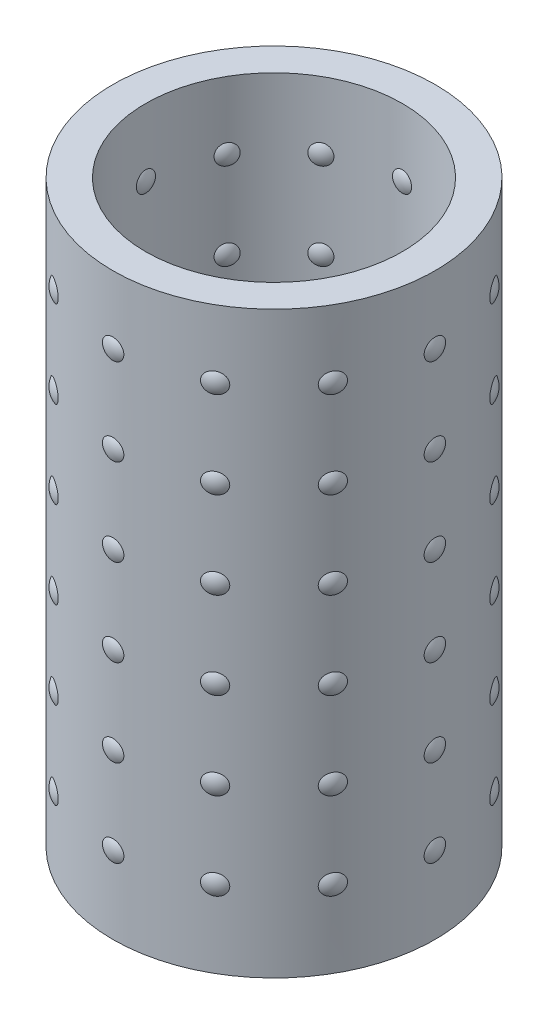
from build123d import *

# Parameters (mm, degrees)
SKETCH1_R           = 8.35
SKETCH1_R_2         = 6.65
BOSS_EXTRUDE1_DEPTH = 30
LPATTERN5_COUNT     = 8
LPATTERN5_PITCH     = 4.5
CIRPATTERN1_COUNT   = 12


with BuildPart() as part:
    # Sketch1 → Boss-Extrude1 (new body)
    with BuildSketch(Plane(origin=(0, 0, 0), x_dir=(1, 0, 0), z_dir=(0, 1, 0))):
        with Locations(Location((0, 0, 0), (0, 0, 270))):
            Circle(SKETCH1_R)
        with Locations(Location((0, 0, 0), (0, 0, 270))):
            Circle(SKETCH1_R_2, mode=Mode.SUBTRACT)
    extrude(amount=BOSS_EXTRUDE1_DEPTH)

    # Sketch2 → Revolve3 (revolve)
    with BuildSketch(Plane(origin=(0, 0, 0), x_dir=(0, 0, -1), z_dir=(1, 0, 0))):
        with BuildLine():
            Line((-8.5, 4), (-6.5, 4))
            ThreePointArc((-6.5, 4), (-7.5, 5), (-8.5, 4))
        make_face()
    revolve3 = revolve(axis=Axis((0, 4, 8.5), (0, 0, -1)))

    # LPattern5: Revolve3 ×8, 2 skipped
    with Locations(*[(0, i * LPATTERN5_PITCH, 0) for i in range(1, LPATTERN5_COUNT) if i not in (6, 7)]):
        add(revolve3)

    # CirPattern1: Revolve3 ×12 about axis
    cirpattern1_axis = Axis((0, 0, 0), (0, 1, 0))
    for i in range(1, CIRPATTERN1_COUNT):
        add(revolve3.rotate(cirpattern1_axis, i * 360 / CIRPATTERN1_COUNT))

    # CirPattern1 copy 1 sketch → CirPattern1 copy 1 (revolve)
    with BuildSketch(Plane(origin=(0, 4.5, 0), x_dir=(-0.49999999999999994, 0, -0.8660254037844387), z_dir=(0.8660254037844387, 0, -0.49999999999999994))):
        with BuildLine():
            Line((-8.5, 4), (-6.5, 4))
            ThreePointArc((-6.5, 4), (-7.5, 5), (-8.5, 4))
        make_face()
    revolve(axis=Axis((4.25, 8.5, 7.361215932), (-0.49999999999999994, 0, -0.8660254037844387)))

    # CirPattern1 copy 2 sketch → CirPattern1 copy 2 (revolve)
    with BuildSketch(Plane(origin=(0, 4.5, 0), x_dir=(-0.8660254037844386, 0, -0.5000000000000001), z_dir=(0.5000000000000001, 0, -0.8660254037844386))):
        with BuildLine():
            Line((-8.5, 4), (-6.5, 4))
            ThreePointArc((-6.5, 4), (-7.5, 5), (-8.5, 4))
        make_face()
    revolve(axis=Axis((7.361215932, 8.5, 4.25), (-0.8660254037844386, 0, -0.5000000000000001)))

    # CirPattern1 copy 3 sketch → CirPattern1 copy 3 (revolve)
    with BuildSketch(Plane(origin=(0, 4.5, 0), x_dir=(-1, 0, 0), z_dir=(0, 0, -1))):
        with BuildLine():
            Line((-8.5, 4), (-6.5, 4))
            ThreePointArc((-6.5, 4), (-7.5, 5), (-8.5, 4))
        make_face()
    revolve(axis=Axis((8.5, 8.5, 0), (-1, 0, 0)))

    # CirPattern1 copy 4 sketch → CirPattern1 copy 4 (revolve)
    with BuildSketch(Plane(origin=(0, 4.5, 0), x_dir=(-0.8660254037844387, 0, 0.4999999999999998), z_dir=(-0.4999999999999998, 0, -0.8660254037844387))):
        with BuildLine():
            Line((-8.5, 4), (-6.5, 4))
            ThreePointArc((-6.5, 4), (-7.5, 5), (-8.5, 4))
        make_face()
    revolve(axis=Axis((7.361215932, 8.5, -4.25), (-0.8660254037844387, 0, 0.4999999999999998)))

    # CirPattern1 copy 5 sketch → CirPattern1 copy 5 (revolve)
    with BuildSketch(Plane(origin=(0, 4.5, 0), x_dir=(-0.49999999999999994, 0, 0.8660254037844387), z_dir=(-0.8660254037844387, 0, -0.49999999999999994))):
        with BuildLine():
            Line((-8.5, 4), (-6.5, 4))
            ThreePointArc((-6.5, 4), (-7.5, 5), (-8.5, 4))
        make_face()
    revolve(axis=Axis((4.25, 8.5, -7.361215932), (-0.49999999999999994, 0, 0.8660254037844387)))

    # CirPattern1 copy 6 sketch → CirPattern1 copy 6 (revolve)
    with BuildSketch(Plane(origin=(0, 4.5, 0), x_dir=(0, 0, 1), z_dir=(-1, 0, 0))):
        with BuildLine():
            Line((-8.5, 4), (-6.5, 4))
            ThreePointArc((-6.5, 4), (-7.5, 5), (-8.5, 4))
        make_face()
    revolve(axis=Axis((0, 8.5, -8.5), (0, 0, 1)))

    # CirPattern1 copy 7 sketch → CirPattern1 copy 7 (revolve)
    with BuildSketch(Plane(origin=(0, 4.5, 0), x_dir=(0.5000000000000001, 0, 0.8660254037844386), z_dir=(-0.8660254037844386, 0, 0.5000000000000001))):
        with BuildLine():
            Line((-8.5, 4), (-6.5, 4))
            ThreePointArc((-6.5, 4), (-7.5, 5), (-8.5, 4))
        make_face()
    revolve(axis=Axis((-4.25, 8.5, -7.361215932), (0.5000000000000001, 0, 0.8660254037844386)))

    # CirPattern1 copy 8 sketch → CirPattern1 copy 8 (revolve)
    with BuildSketch(Plane(origin=(0, 4.5, 0), x_dir=(0.8660254037844384, 0, 0.5000000000000004), z_dir=(-0.5000000000000004, 0, 0.8660254037844384))):
        with BuildLine():
            Line((-8.5, 4), (-6.5, 4))
            ThreePointArc((-6.5, 4), (-7.5, 5), (-8.5, 4))
        make_face()
    revolve(axis=Axis((-7.361215932, 8.5, -4.25), (0.8660254037844384, 0, 0.5000000000000004)))

    # CirPattern1 copy 9 sketch → CirPattern1 copy 9 (revolve)
    with BuildSketch(Plane(origin=(0, 4.5, 0), x_dir=(1, 0, 0), z_dir=(0, 0, 1))):
        with BuildLine():
            Line((-8.5, 4), (-6.5, 4))
            ThreePointArc((-6.5, 4), (-7.5, 5), (-8.5, 4))
        make_face()
    revolve(axis=Axis((-8.5, 8.5, 0), (1, 0, 0)))

    # CirPattern1 copy 10 sketch → CirPattern1 copy 10 (revolve)
    with BuildSketch(Plane(origin=(0, 4.5, 0), x_dir=(0.8660254037844386, 0, -0.5000000000000001), z_dir=(0.5000000000000001, 0, 0.8660254037844386))):
        with BuildLine():
            Line((-8.5, 4), (-6.5, 4))
            ThreePointArc((-6.5, 4), (-7.5, 5), (-8.5, 4))
        make_face()
    revolve(axis=Axis((-7.361215932, 8.5, 4.25), (0.8660254037844386, 0, -0.5000000000000001)))

    # CirPattern1 copy 11 sketch → CirPattern1 copy 11 (revolve)
    with BuildSketch(Plane(origin=(0, 4.5, 0), x_dir=(0.5000000000000004, 0, -0.8660254037844384), z_dir=(0.8660254037844384, 0, 0.5000000000000004))):
        with BuildLine():
            Line((-8.5, 4), (-6.5, 4))
            ThreePointArc((-6.5, 4), (-7.5, 5), (-8.5, 4))
        make_face()
    revolve(axis=Axis((-4.25, 8.5, 7.361215932), (0.5000000000000004, 0, -0.8660254037844384)))

    # CirPattern1 copy 12 sketch → CirPattern1 copy 12 (revolve)
    with BuildSketch(Plane(origin=(0, 9, 0), x_dir=(-0.49999999999999994, 0, -0.8660254037844387), z_dir=(0.8660254037844387, 0, -0.49999999999999994))):
        with BuildLine():
            Line((-8.5, 4), (-6.5, 4))
            ThreePointArc((-6.5, 4), (-7.5, 5), (-8.5, 4))
        make_face()
    revolve(axis=Axis((4.25, 13, 7.361215932), (-0.49999999999999994, 0, -0.8660254037844387)))

    # CirPattern1 copy 13 sketch → CirPattern1 copy 13 (revolve)
    with BuildSketch(Plane(origin=(0, 9, 0), x_dir=(-0.8660254037844386, 0, -0.5000000000000001), z_dir=(0.5000000000000001, 0, -0.8660254037844386))):
        with BuildLine():
            Line((-8.5, 4), (-6.5, 4))
            ThreePointArc((-6.5, 4), (-7.5, 5), (-8.5, 4))
        make_face()
    revolve(axis=Axis((7.361215932, 13, 4.25), (-0.8660254037844386, 0, -0.5000000000000001)))

    # CirPattern1 copy 14 sketch → CirPattern1 copy 14 (revolve)
    with BuildSketch(Plane(origin=(0, 9, 0), x_dir=(-1, 0, 0), z_dir=(0, 0, -1))):
        with BuildLine():
            Line((-8.5, 4), (-6.5, 4))
            ThreePointArc((-6.5, 4), (-7.5, 5), (-8.5, 4))
        make_face()
    revolve(axis=Axis((8.5, 13, 0), (-1, 0, 0)))

    # CirPattern1 copy 15 sketch → CirPattern1 copy 15 (revolve)
    with BuildSketch(Plane(origin=(0, 9, 0), x_dir=(-0.8660254037844387, 0, 0.4999999999999998), z_dir=(-0.4999999999999998, 0, -0.8660254037844387))):
        with BuildLine():
            Line((-8.5, 4), (-6.5, 4))
            ThreePointArc((-6.5, 4), (-7.5, 5), (-8.5, 4))
        make_face()
    revolve(axis=Axis((7.361215932, 13, -4.25), (-0.8660254037844387, 0, 0.4999999999999998)))

    # CirPattern1 copy 16 sketch → CirPattern1 copy 16 (revolve)
    with BuildSketch(Plane(origin=(0, 9, 0), x_dir=(-0.49999999999999994, 0, 0.8660254037844387), z_dir=(-0.8660254037844387, 0, -0.49999999999999994))):
        with BuildLine():
            Line((-8.5, 4), (-6.5, 4))
            ThreePointArc((-6.5, 4), (-7.5, 5), (-8.5, 4))
        make_face()
    revolve(axis=Axis((4.25, 13, -7.361215932), (-0.49999999999999994, 0, 0.8660254037844387)))

    # CirPattern1 copy 17 sketch → CirPattern1 copy 17 (revolve)
    with BuildSketch(Plane(origin=(0, 9, 0), x_dir=(0, 0, 1), z_dir=(-1, 0, 0))):
        with BuildLine():
            Line((-8.5, 4), (-6.5, 4))
            ThreePointArc((-6.5, 4), (-7.5, 5), (-8.5, 4))
        make_face()
    revolve(axis=Axis((0, 13, -8.5), (0, 0, 1)))

    # CirPattern1 copy 18 sketch → CirPattern1 copy 18 (revolve)
    with BuildSketch(Plane(origin=(0, 9, 0), x_dir=(0.5000000000000001, 0, 0.8660254037844386), z_dir=(-0.8660254037844386, 0, 0.5000000000000001))):
        with BuildLine():
            Line((-8.5, 4), (-6.5, 4))
            ThreePointArc((-6.5, 4), (-7.5, 5), (-8.5, 4))
        make_face()
    revolve(axis=Axis((-4.25, 13, -7.361215932), (0.5000000000000001, 0, 0.8660254037844386)))

    # CirPattern1 copy 19 sketch → CirPattern1 copy 19 (revolve)
    with BuildSketch(Plane(origin=(0, 9, 0), x_dir=(0.8660254037844384, 0, 0.5000000000000004), z_dir=(-0.5000000000000004, 0, 0.8660254037844384))):
        with BuildLine():
            Line((-8.5, 4), (-6.5, 4))
            ThreePointArc((-6.5, 4), (-7.5, 5), (-8.5, 4))
        make_face()
    revolve(axis=Axis((-7.361215932, 13, -4.25), (0.8660254037844384, 0, 0.5000000000000004)))

    # CirPattern1 copy 20 sketch → CirPattern1 copy 20 (revolve)
    with BuildSketch(Plane(origin=(0, 9, 0), x_dir=(1, 0, 0), z_dir=(0, 0, 1))):
        with BuildLine():
            Line((-8.5, 4), (-6.5, 4))
            ThreePointArc((-6.5, 4), (-7.5, 5), (-8.5, 4))
        make_face()
    revolve(axis=Axis((-8.5, 13, 0), (1, 0, 0)))

    # CirPattern1 copy 21 sketch → CirPattern1 copy 21 (revolve)
    with BuildSketch(Plane(origin=(0, 9, 0), x_dir=(0.8660254037844386, 0, -0.5000000000000001), z_dir=(0.5000000000000001, 0, 0.8660254037844386))):
        with BuildLine():
            Line((-8.5, 4), (-6.5, 4))
            ThreePointArc((-6.5, 4), (-7.5, 5), (-8.5, 4))
        make_face()
    revolve(axis=Axis((-7.361215932, 13, 4.25), (0.8660254037844386, 0, -0.5000000000000001)))

    # CirPattern1 copy 22 sketch → CirPattern1 copy 22 (revolve)
    with BuildSketch(Plane(origin=(0, 9, 0), x_dir=(0.5000000000000004, 0, -0.8660254037844384), z_dir=(0.8660254037844384, 0, 0.5000000000000004))):
        with BuildLine():
            Line((-8.5, 4), (-6.5, 4))
            ThreePointArc((-6.5, 4), (-7.5, 5), (-8.5, 4))
        make_face()
    revolve(axis=Axis((-4.25, 13, 7.361215932), (0.5000000000000004, 0, -0.8660254037844384)))

    # CirPattern1 copy 23 sketch → CirPattern1 copy 23 (revolve)
    with BuildSketch(Plane(origin=(0, 13.5, 0), x_dir=(-0.49999999999999994, 0, -0.8660254037844387), z_dir=(0.8660254037844387, 0, -0.49999999999999994))):
        with BuildLine():
            Line((-8.5, 4), (-6.5, 4))
            ThreePointArc((-6.5, 4), (-7.5, 5), (-8.5, 4))
        make_face()
    revolve(axis=Axis((4.25, 17.5, 7.361215932), (-0.49999999999999994, 0, -0.8660254037844387)))

    # CirPattern1 copy 24 sketch → CirPattern1 copy 24 (revolve)
    with BuildSketch(Plane(origin=(0, 13.5, 0), x_dir=(-0.8660254037844386, 0, -0.5000000000000001), z_dir=(0.5000000000000001, 0, -0.8660254037844386))):
        with BuildLine():
            Line((-8.5, 4), (-6.5, 4))
            ThreePointArc((-6.5, 4), (-7.5, 5), (-8.5, 4))
        make_face()
    revolve(axis=Axis((7.361215932, 17.5, 4.25), (-0.8660254037844386, 0, -0.5000000000000001)))

    # CirPattern1 copy 25 sketch → CirPattern1 copy 25 (revolve)
    with BuildSketch(Plane(origin=(0, 13.5, 0), x_dir=(-1, 0, 0), z_dir=(0, 0, -1))):
        with BuildLine():
            Line((-8.5, 4), (-6.5, 4))
            ThreePointArc((-6.5, 4), (-7.5, 5), (-8.5, 4))
        make_face()
    revolve(axis=Axis((8.5, 17.5, 0), (-1, 0, 0)))

    # CirPattern1 copy 26 sketch → CirPattern1 copy 26 (revolve)
    with BuildSketch(Plane(origin=(0, 13.5, 0), x_dir=(-0.8660254037844387, 0, 0.4999999999999998), z_dir=(-0.4999999999999998, 0, -0.8660254037844387))):
        with BuildLine():
            Line((-8.5, 4), (-6.5, 4))
            ThreePointArc((-6.5, 4), (-7.5, 5), (-8.5, 4))
        make_face()
    revolve(axis=Axis((7.361215932, 17.5, -4.25), (-0.8660254037844387, 0, 0.4999999999999998)))

    # CirPattern1 copy 27 sketch → CirPattern1 copy 27 (revolve)
    with BuildSketch(Plane(origin=(0, 13.5, 0), x_dir=(-0.49999999999999994, 0, 0.8660254037844387), z_dir=(-0.8660254037844387, 0, -0.49999999999999994))):
        with BuildLine():
            Line((-8.5, 4), (-6.5, 4))
            ThreePointArc((-6.5, 4), (-7.5, 5), (-8.5, 4))
        make_face()
    revolve(axis=Axis((4.25, 17.5, -7.361215932), (-0.49999999999999994, 0, 0.8660254037844387)))

    # CirPattern1 copy 28 sketch → CirPattern1 copy 28 (revolve)
    with BuildSketch(Plane(origin=(0, 13.5, 0), x_dir=(0, 0, 1), z_dir=(-1, 0, 0))):
        with BuildLine():
            Line((-8.5, 4), (-6.5, 4))
            ThreePointArc((-6.5, 4), (-7.5, 5), (-8.5, 4))
        make_face()
    revolve(axis=Axis((0, 17.5, -8.5), (0, 0, 1)))

    # CirPattern1 copy 29 sketch → CirPattern1 copy 29 (revolve)
    with BuildSketch(Plane(origin=(0, 13.5, 0), x_dir=(0.5000000000000001, 0, 0.8660254037844386), z_dir=(-0.8660254037844386, 0, 0.5000000000000001))):
        with BuildLine():
            Line((-8.5, 4), (-6.5, 4))
            ThreePointArc((-6.5, 4), (-7.5, 5), (-8.5, 4))
        make_face()
    revolve(axis=Axis((-4.25, 17.5, -7.361215932), (0.5000000000000001, 0, 0.8660254037844386)))

    # CirPattern1 copy 30 sketch → CirPattern1 copy 30 (revolve)
    with BuildSketch(Plane(origin=(0, 13.5, 0), x_dir=(0.8660254037844384, 0, 0.5000000000000004), z_dir=(-0.5000000000000004, 0, 0.8660254037844384))):
        with BuildLine():
            Line((-8.5, 4), (-6.5, 4))
            ThreePointArc((-6.5, 4), (-7.5, 5), (-8.5, 4))
        make_face()
    revolve(axis=Axis((-7.361215932, 17.5, -4.25), (0.8660254037844384, 0, 0.5000000000000004)))

    # CirPattern1 copy 31 sketch → CirPattern1 copy 31 (revolve)
    with BuildSketch(Plane(origin=(0, 13.5, 0), x_dir=(1, 0, 0), z_dir=(0, 0, 1))):
        with BuildLine():
            Line((-8.5, 4), (-6.5, 4))
            ThreePointArc((-6.5, 4), (-7.5, 5), (-8.5, 4))
        make_face()
    revolve(axis=Axis((-8.5, 17.5, 0), (1, 0, 0)))

    # CirPattern1 copy 32 sketch → CirPattern1 copy 32 (revolve)
    with BuildSketch(Plane(origin=(0, 13.5, 0), x_dir=(0.8660254037844386, 0, -0.5000000000000001), z_dir=(0.5000000000000001, 0, 0.8660254037844386))):
        with BuildLine():
            Line((-8.5, 4), (-6.5, 4))
            ThreePointArc((-6.5, 4), (-7.5, 5), (-8.5, 4))
        make_face()
    revolve(axis=Axis((-7.361215932, 17.5, 4.25), (0.8660254037844386, 0, -0.5000000000000001)))

    # CirPattern1 copy 33 sketch → CirPattern1 copy 33 (revolve)
    with BuildSketch(Plane(origin=(0, 13.5, 0), x_dir=(0.5000000000000004, 0, -0.8660254037844384), z_dir=(0.8660254037844384, 0, 0.5000000000000004))):
        with BuildLine():
            Line((-8.5, 4), (-6.5, 4))
            ThreePointArc((-6.5, 4), (-7.5, 5), (-8.5, 4))
        make_face()
    revolve(axis=Axis((-4.25, 17.5, 7.361215932), (0.5000000000000004, 0, -0.8660254037844384)))

    # CirPattern1 copy 34 sketch → CirPattern1 copy 34 (revolve)
    with BuildSketch(Plane(origin=(0, 18, 0), x_dir=(-0.49999999999999994, 0, -0.8660254037844387), z_dir=(0.8660254037844387, 0, -0.49999999999999994))):
        with BuildLine():
            Line((-8.5, 4), (-6.5, 4))
            ThreePointArc((-6.5, 4), (-7.5, 5), (-8.5, 4))
        make_face()
    revolve(axis=Axis((4.25, 22, 7.361215932), (-0.49999999999999994, 0, -0.8660254037844387)))

    # CirPattern1 copy 35 sketch → CirPattern1 copy 35 (revolve)
    with BuildSketch(Plane(origin=(0, 18, 0), x_dir=(-0.8660254037844386, 0, -0.5000000000000001), z_dir=(0.5000000000000001, 0, -0.8660254037844386))):
        with BuildLine():
            Line((-8.5, 4), (-6.5, 4))
            ThreePointArc((-6.5, 4), (-7.5, 5), (-8.5, 4))
        make_face()
    revolve(axis=Axis((7.361215932, 22, 4.25), (-0.8660254037844386, 0, -0.5000000000000001)))

    # CirPattern1 copy 36 sketch → CirPattern1 copy 36 (revolve)
    with BuildSketch(Plane(origin=(0, 18, 0), x_dir=(-1, 0, 0), z_dir=(0, 0, -1))):
        with BuildLine():
            Line((-8.5, 4), (-6.5, 4))
            ThreePointArc((-6.5, 4), (-7.5, 5), (-8.5, 4))
        make_face()
    revolve(axis=Axis((8.5, 22, 0), (-1, 0, 0)))

    # CirPattern1 copy 37 sketch → CirPattern1 copy 37 (revolve)
    with BuildSketch(Plane(origin=(0, 18, 0), x_dir=(-0.8660254037844387, 0, 0.4999999999999998), z_dir=(-0.4999999999999998, 0, -0.8660254037844387))):
        with BuildLine():
            Line((-8.5, 4), (-6.5, 4))
            ThreePointArc((-6.5, 4), (-7.5, 5), (-8.5, 4))
        make_face()
    revolve(axis=Axis((7.361215932, 22, -4.25), (-0.8660254037844387, 0, 0.4999999999999998)))

    # CirPattern1 copy 38 sketch → CirPattern1 copy 38 (revolve)
    with BuildSketch(Plane(origin=(0, 18, 0), x_dir=(-0.49999999999999994, 0, 0.8660254037844387), z_dir=(-0.8660254037844387, 0, -0.49999999999999994))):
        with BuildLine():
            Line((-8.5, 4), (-6.5, 4))
            ThreePointArc((-6.5, 4), (-7.5, 5), (-8.5, 4))
        make_face()
    revolve(axis=Axis((4.25, 22, -7.361215932), (-0.49999999999999994, 0, 0.8660254037844387)))

    # CirPattern1 copy 39 sketch → CirPattern1 copy 39 (revolve)
    with BuildSketch(Plane(origin=(0, 18, 0), x_dir=(0, 0, 1), z_dir=(-1, 0, 0))):
        with BuildLine():
            Line((-8.5, 4), (-6.5, 4))
            ThreePointArc((-6.5, 4), (-7.5, 5), (-8.5, 4))
        make_face()
    revolve(axis=Axis((0, 22, -8.5), (0, 0, 1)))

    # CirPattern1 copy 40 sketch → CirPattern1 copy 40 (revolve)
    with BuildSketch(Plane(origin=(0, 18, 0), x_dir=(0.5000000000000001, 0, 0.8660254037844386), z_dir=(-0.8660254037844386, 0, 0.5000000000000001))):
        with BuildLine():
            Line((-8.5, 4), (-6.5, 4))
            ThreePointArc((-6.5, 4), (-7.5, 5), (-8.5, 4))
        make_face()
    revolve(axis=Axis((-4.25, 22, -7.361215932), (0.5000000000000001, 0, 0.8660254037844386)))

    # CirPattern1 copy 41 sketch → CirPattern1 copy 41 (revolve)
    with BuildSketch(Plane(origin=(0, 18, 0), x_dir=(0.8660254037844384, 0, 0.5000000000000004), z_dir=(-0.5000000000000004, 0, 0.8660254037844384))):
        with BuildLine():
            Line((-8.5, 4), (-6.5, 4))
            ThreePointArc((-6.5, 4), (-7.5, 5), (-8.5, 4))
        make_face()
    revolve(axis=Axis((-7.361215932, 22, -4.25), (0.8660254037844384, 0, 0.5000000000000004)))

    # CirPattern1 copy 42 sketch → CirPattern1 copy 42 (revolve)
    with BuildSketch(Plane(origin=(0, 18, 0), x_dir=(1, 0, 0), z_dir=(0, 0, 1))):
        with BuildLine():
            Line((-8.5, 4), (-6.5, 4))
            ThreePointArc((-6.5, 4), (-7.5, 5), (-8.5, 4))
        make_face()
    revolve(axis=Axis((-8.5, 22, 0), (1, 0, 0)))

    # CirPattern1 copy 43 sketch → CirPattern1 copy 43 (revolve)
    with BuildSketch(Plane(origin=(0, 18, 0), x_dir=(0.8660254037844386, 0, -0.5000000000000001), z_dir=(0.5000000000000001, 0, 0.8660254037844386))):
        with BuildLine():
            Line((-8.5, 4), (-6.5, 4))
            ThreePointArc((-6.5, 4), (-7.5, 5), (-8.5, 4))
        make_face()
    revolve(axis=Axis((-7.361215932, 22, 4.25), (0.8660254037844386, 0, -0.5000000000000001)))

    # CirPattern1 copy 44 sketch → CirPattern1 copy 44 (revolve)
    with BuildSketch(Plane(origin=(0, 18, 0), x_dir=(0.5000000000000004, 0, -0.8660254037844384), z_dir=(0.8660254037844384, 0, 0.5000000000000004))):
        with BuildLine():
            Line((-8.5, 4), (-6.5, 4))
            ThreePointArc((-6.5, 4), (-7.5, 5), (-8.5, 4))
        make_face()
    revolve(axis=Axis((-4.25, 22, 7.361215932), (0.5000000000000004, 0, -0.8660254037844384)))

    # CirPattern1 copy 45 sketch → CirPattern1 copy 45 (revolve)
    with BuildSketch(Plane(origin=(0, 22.5, 0), x_dir=(-0.49999999999999994, 0, -0.8660254037844387), z_dir=(0.8660254037844387, 0, -0.49999999999999994))):
        with BuildLine():
            Line((-8.5, 4), (-6.5, 4))
            ThreePointArc((-6.5, 4), (-7.5, 5), (-8.5, 4))
        make_face()
    revolve(axis=Axis((4.25, 26.5, 7.361215932), (-0.49999999999999994, 0, -0.8660254037844387)))

    # CirPattern1 copy 46 sketch → CirPattern1 copy 46 (revolve)
    with BuildSketch(Plane(origin=(0, 22.5, 0), x_dir=(-0.8660254037844386, 0, -0.5000000000000001), z_dir=(0.5000000000000001, 0, -0.8660254037844386))):
        with BuildLine():
            Line((-8.5, 4), (-6.5, 4))
            ThreePointArc((-6.5, 4), (-7.5, 5), (-8.5, 4))
        make_face()
    revolve(axis=Axis((7.361215932, 26.5, 4.25), (-0.8660254037844386, 0, -0.5000000000000001)))

    # CirPattern1 copy 47 sketch → CirPattern1 copy 47 (revolve)
    with BuildSketch(Plane(origin=(0, 22.5, 0), x_dir=(-1, 0, 0), z_dir=(0, 0, -1))):
        with BuildLine():
            Line((-8.5, 4), (-6.5, 4))
            ThreePointArc((-6.5, 4), (-7.5, 5), (-8.5, 4))
        make_face()
    revolve(axis=Axis((8.5, 26.5, 0), (-1, 0, 0)))

    # CirPattern1 copy 48 sketch → CirPattern1 copy 48 (revolve)
    with BuildSketch(Plane(origin=(0, 22.5, 0), x_dir=(-0.8660254037844387, 0, 0.4999999999999998), z_dir=(-0.4999999999999998, 0, -0.8660254037844387))):
        with BuildLine():
            Line((-8.5, 4), (-6.5, 4))
            ThreePointArc((-6.5, 4), (-7.5, 5), (-8.5, 4))
        make_face()
    revolve(axis=Axis((7.361215932, 26.5, -4.25), (-0.8660254037844387, 0, 0.4999999999999998)))

    # CirPattern1 copy 49 sketch → CirPattern1 copy 49 (revolve)
    with BuildSketch(Plane(origin=(0, 22.5, 0), x_dir=(-0.49999999999999994, 0, 0.8660254037844387), z_dir=(-0.8660254037844387, 0, -0.49999999999999994))):
        with BuildLine():
            Line((-8.5, 4), (-6.5, 4))
            ThreePointArc((-6.5, 4), (-7.5, 5), (-8.5, 4))
        make_face()
    revolve(axis=Axis((4.25, 26.5, -7.361215932), (-0.49999999999999994, 0, 0.8660254037844387)))

    # CirPattern1 copy 50 sketch → CirPattern1 copy 50 (revolve)
    with BuildSketch(Plane(origin=(0, 22.5, 0), x_dir=(0, 0, 1), z_dir=(-1, 0, 0))):
        with BuildLine():
            Line((-8.5, 4), (-6.5, 4))
            ThreePointArc((-6.5, 4), (-7.5, 5), (-8.5, 4))
        make_face()
    revolve(axis=Axis((0, 26.5, -8.5), (0, 0, 1)))

    # CirPattern1 copy 51 sketch → CirPattern1 copy 51 (revolve)
    with BuildSketch(Plane(origin=(0, 22.5, 0), x_dir=(0.5000000000000001, 0, 0.8660254037844386), z_dir=(-0.8660254037844386, 0, 0.5000000000000001))):
        with BuildLine():
            Line((-8.5, 4), (-6.5, 4))
            ThreePointArc((-6.5, 4), (-7.5, 5), (-8.5, 4))
        make_face()
    revolve(axis=Axis((-4.25, 26.5, -7.361215932), (0.5000000000000001, 0, 0.8660254037844386)))

    # CirPattern1 copy 52 sketch → CirPattern1 copy 52 (revolve)
    with BuildSketch(Plane(origin=(0, 22.5, 0), x_dir=(0.8660254037844384, 0, 0.5000000000000004), z_dir=(-0.5000000000000004, 0, 0.8660254037844384))):
        with BuildLine():
            Line((-8.5, 4), (-6.5, 4))
            ThreePointArc((-6.5, 4), (-7.5, 5), (-8.5, 4))
        make_face()
    revolve(axis=Axis((-7.361215932, 26.5, -4.25), (0.8660254037844384, 0, 0.5000000000000004)))

    # CirPattern1 copy 53 sketch → CirPattern1 copy 53 (revolve)
    with BuildSketch(Plane(origin=(0, 22.5, 0), x_dir=(1, 0, 0), z_dir=(0, 0, 1))):
        with BuildLine():
            Line((-8.5, 4), (-6.5, 4))
            ThreePointArc((-6.5, 4), (-7.5, 5), (-8.5, 4))
        make_face()
    revolve(axis=Axis((-8.5, 26.5, 0), (1, 0, 0)))

    # CirPattern1 copy 54 sketch → CirPattern1 copy 54 (revolve)
    with BuildSketch(Plane(origin=(0, 22.5, 0), x_dir=(0.8660254037844386, 0, -0.5000000000000001), z_dir=(0.5000000000000001, 0, 0.8660254037844386))):
        with BuildLine():
            Line((-8.5, 4), (-6.5, 4))
            ThreePointArc((-6.5, 4), (-7.5, 5), (-8.5, 4))
        make_face()
    revolve(axis=Axis((-7.361215932, 26.5, 4.25), (0.8660254037844386, 0, -0.5000000000000001)))

    # CirPattern1 copy 55 sketch → CirPattern1 copy 55 (revolve)
    with BuildSketch(Plane(origin=(0, 22.5, 0), x_dir=(0.5000000000000004, 0, -0.8660254037844384), z_dir=(0.8660254037844384, 0, 0.5000000000000004))):
        with BuildLine():
            Line((-8.5, 4), (-6.5, 4))
            ThreePointArc((-6.5, 4), (-7.5, 5), (-8.5, 4))
        make_face()
    revolve(axis=Axis((-4.25, 26.5, 7.361215932), (0.5000000000000004, 0, -0.8660254037844384)))


solid = part.part
